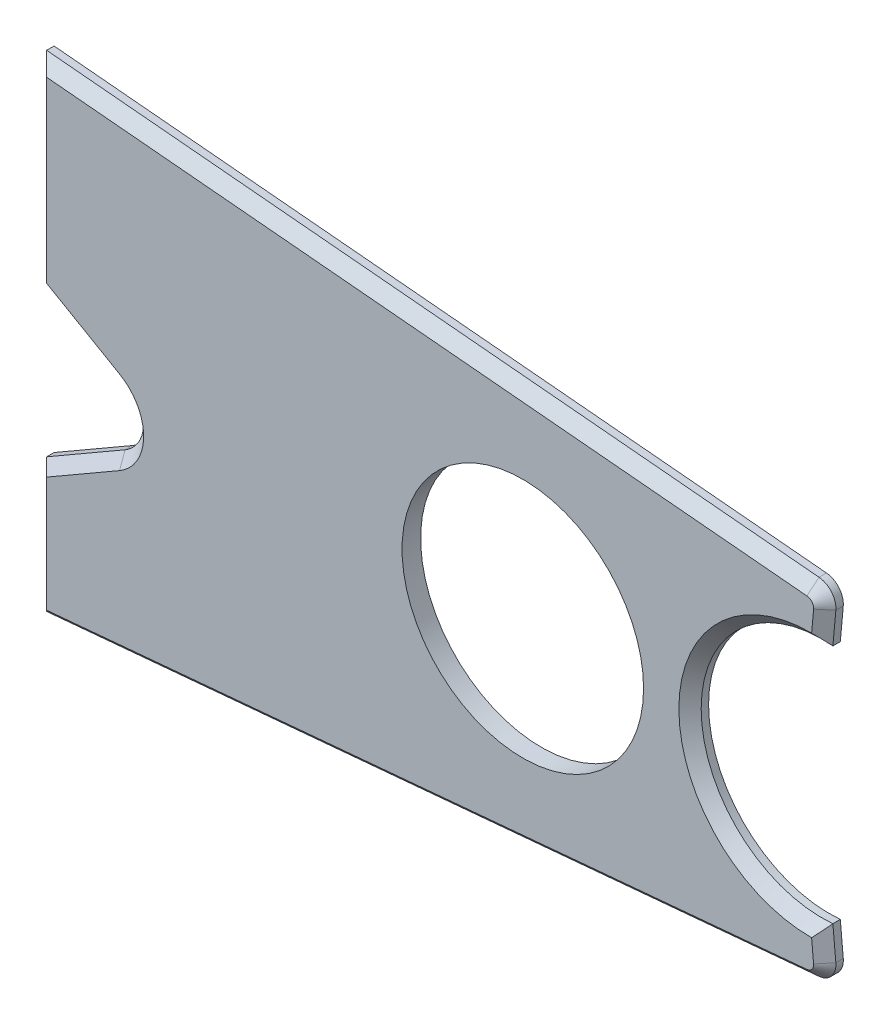
SolidWorks part; units mm, degrees
ref_plane "Front Plane" through (0, 0, 0) normal (0, 0, 1) x (1, 0, 0)
ref_plane "Top Plane" through (0, 0, 0) normal (0, 1, 0) x (1, 0, 0)
ref_plane "Right Plane" through (0, 0, 0) normal (1, 0, 0) x (0, 0, -1)
sketch "Sketch1" plane through (0, 0, 0) normal (0, 0, 1) x (1, 0, 0)
  line L0 (-94.5847, 0) -> (177.0221, 0) construction
  line L1 (155, 125.9672) -> (155, -105.1174) construction
  line L2 (-262.3, 130.8) -> (-262.3, 24.7)
  line L3 (-262.3, 130.8) -> (153.441, 93.0228)
  line L4 (-262.3, -130.8) -> (153.441, -93.0228)
  line L5 (162.4951, 82.1588) -> (160.9114, 64.7306)
  line L6 (162.4951, -82.1588) -> (160.9114, -64.7306)
  line L9 (-262.3, -58.7) -> (-220.0735, -34.3205)
  line L10 (-262.3, 24.7) -> (-220.0735, 0.3205)
  line L11 (-262.3, -58.7) -> (-262.3, -130.8)
  circle A0 centre (0, 0) radius 65
  arc A1 (160.9114, 64.7306) -> (160.9114, -64.7306) centre (155, 0) ccw
  arc A2 (-220.0735, 0.3205) -> (-220.0735, -34.3205) centre (-230.0735, -17) cw
  arc A3 (163.3707, -92.1205) -> (163.3707, 92.1205) centre (155, 0) ccw construction
  arc A4 (153.441, -93.0228) -> (162.4951, -82.1588) centre (152.5361, -83.0638) ccw
  arc A5 (153.441, 93.0228) -> (162.4951, 82.1588) centre (152.5361, 83.0638) cw
  point P24 (163.4, -92.1178)
  point P27 (163.4, 92.1178)
  dimension "D1" = 130
  dimension "D3" = 130
  dimension "D17" = 20
  dimension "D7" = 185
  dimension "D5" = 10
  dimension "D2" = 155
  dimension "D4" = 262.3
  dimension "D6" = 261.6
  dimension "D8" = 8.4
  dimension "D13" = 72.1
  dimension "D14" = 83.4
  dimension "D15" = 60
  dimension "D16" = 30
extrude "Boss-Extrude1" add sketch "Sketch1" along normal blind 10
chamfer "Chamfer1" distance 6 angle 45 12 edges at (-54.4295, -111.9114, 10) (-262.3, -94.75, 10) (-241.1867, -46.5103, 10) (-210.0735, -17, 10) (-241.1867, 12.5103, 10) (-262.3, 77.75, 10) (-54.4295, 111.9114, 10) (161.7032, -73.4447, 10) (90, 0, 10) (161.7032, 73.4447, 10) (160.218, -89.4659, 10) (160.218, 89.4659, 10)
